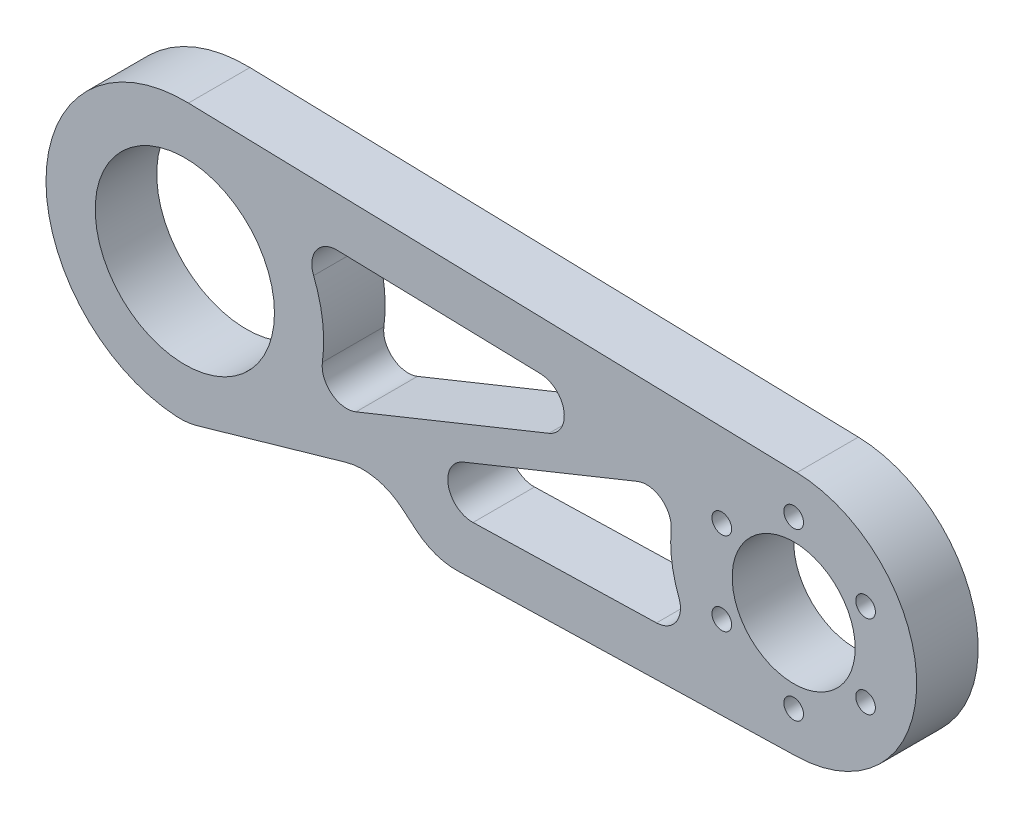
SolidWorks part; units mm, degrees
material "哈碳纤"
ref_plane "前视基准面" through (0, 0, 0) normal (0, 0, 1) x (1, 0, 0)
ref_plane "上视基准面" through (0, 0, 0) normal (0, 1, 0) x (1, 0, 0)
ref_plane "右视基准面" through (0, 0, 0) normal (1, 0, 0) x (0, 0, -1)
other "Configuration Table"
sketch "草图1" plane through (0, 0, 0) normal (0, 0, 1) x (1, 0, 0)
  line L0 (0, 0) -> (99, 0) construction
  line L1 (0.5872, 22.5674) -> (99.5202, 19.9932)
  line L2 (0.5872, -22.5674) -> (99.5202, -19.9932)
  circle A0 centre (0, 0) radius 14.575
  circle A1 centre (0, 0) radius 22.575
  circle A2 centre (99, 0) radius 10
  circle A3 centre (99, 0) radius 20
  dimension "D2" = 29.15
  dimension "D3" = 8
  dimension "D4" = 20
  dimension "D5" = 10
  dimension "D1" = 99
extrude "凸台-拉伸1" add sketch "草图1" along normal blind 10
sketch "草图2" plane through (0, 0, 10) normal (0, 0, 1) x (1, 0, 0)
  line L2 (0.3791, 14.5701) -> (99.3121, 11.9959)
  line L3 (0.3791, 14.5701) -> (99.3121, 11.9959)
  line L4 (17.6128, -14.1217) -> (83.3175, 12.4121)
  line L5 (0.3791, -14.5701) -> (99.3121, -11.9959)
  line L6 (0.3791, -14.5701) -> (99.3121, -11.9959)
  line L7 (18.5489, -16.4398) -> (84.2537, 10.094)
  line L8 (16.6766, -11.8036) -> (82.3814, 14.7302)
  circle A0 centre (0, 0) radius 22.575
  circle A1 centre (99, 0) radius 20
  arc A2 (99.5202, -19.9932) -> (99.5202, 19.9932) centre (99, 0) ccw construction
  dimension "D3" = 45.15
  dimension "D1" = 8
  dimension "D2" = 8
  dimension "D5" = 2.5
  dimension "D6" = 2.5
extrude "切除-拉伸1" cut sketch "草图2" against normal blind 10 contours A0 L8 L3 | A1 L7 L6
fillet "圆角1" radius 4 6 edges at (83.3175, -12.4121, 5) (24.7489, -13.936, 5) (81.0377, 8.7953, 5) (77.0452, 12.5753, 5) (20.006, -10.4591, 5) (17.6128, 14.1217, 5)
ref_plane "基准面1" through (0, 0, 0) normal (0, -1, 0) x (-1, 0, 0)
sketch "草图3" plane through (0, 0, 10) normal (0, 0, 1) x (1, 0, 0)
  circle A0 centre (99, 0) radius 13.5 construction
  arc A1 (99.5202, -19.9932) -> (99.5202, 19.9932) centre (99, 0) ccw construction
  circle A2 centre (99, 13.5) radius 1.6
  circle A3 centre (110.6913, 6.75) radius 1.6
  circle A4 centre (110.6913, -6.75) radius 1.6
  circle A5 centre (99, -13.5) radius 1.6
  circle A6 centre (87.3087, -6.75) radius 1.6
  circle A7 centre (87.3087, 6.75) radius 1.6
  point P21 (99, 0)
  dimension "D1" = 27
  dimension "3.2" = 3.2
  dimension "D3" = 6
extrude "切除-拉伸2" cut sketch "草图3" against normal blind 10
sketch "草图4" plane through (0, 0, 10) normal (0, 0, 1) x (1, 0, 0)
  line L0 (0.5872, -22.5674) -> (31.3023, -13.7655)
  line L1 (31.3023, -13.7655) -> (40.5872, -21.5266)
  line L2 (0.5872, -22.5674) -> (99.5202, -19.9932) construction
  line L3 (0.5872, -22.5674) -> (40.5872, -21.5266)
  dimension "D1" = 8
  dimension "D2" = 40
  dimension "D3" = 14.5
extrude "切除-拉伸3" cut sketch "草图4" against normal blind 10
fillet "圆角2" radius 10 3 edges at (0.5872, -22.5674, 5) (31.3023, -13.7655, 5) (40.5872, -21.5266, 5)
